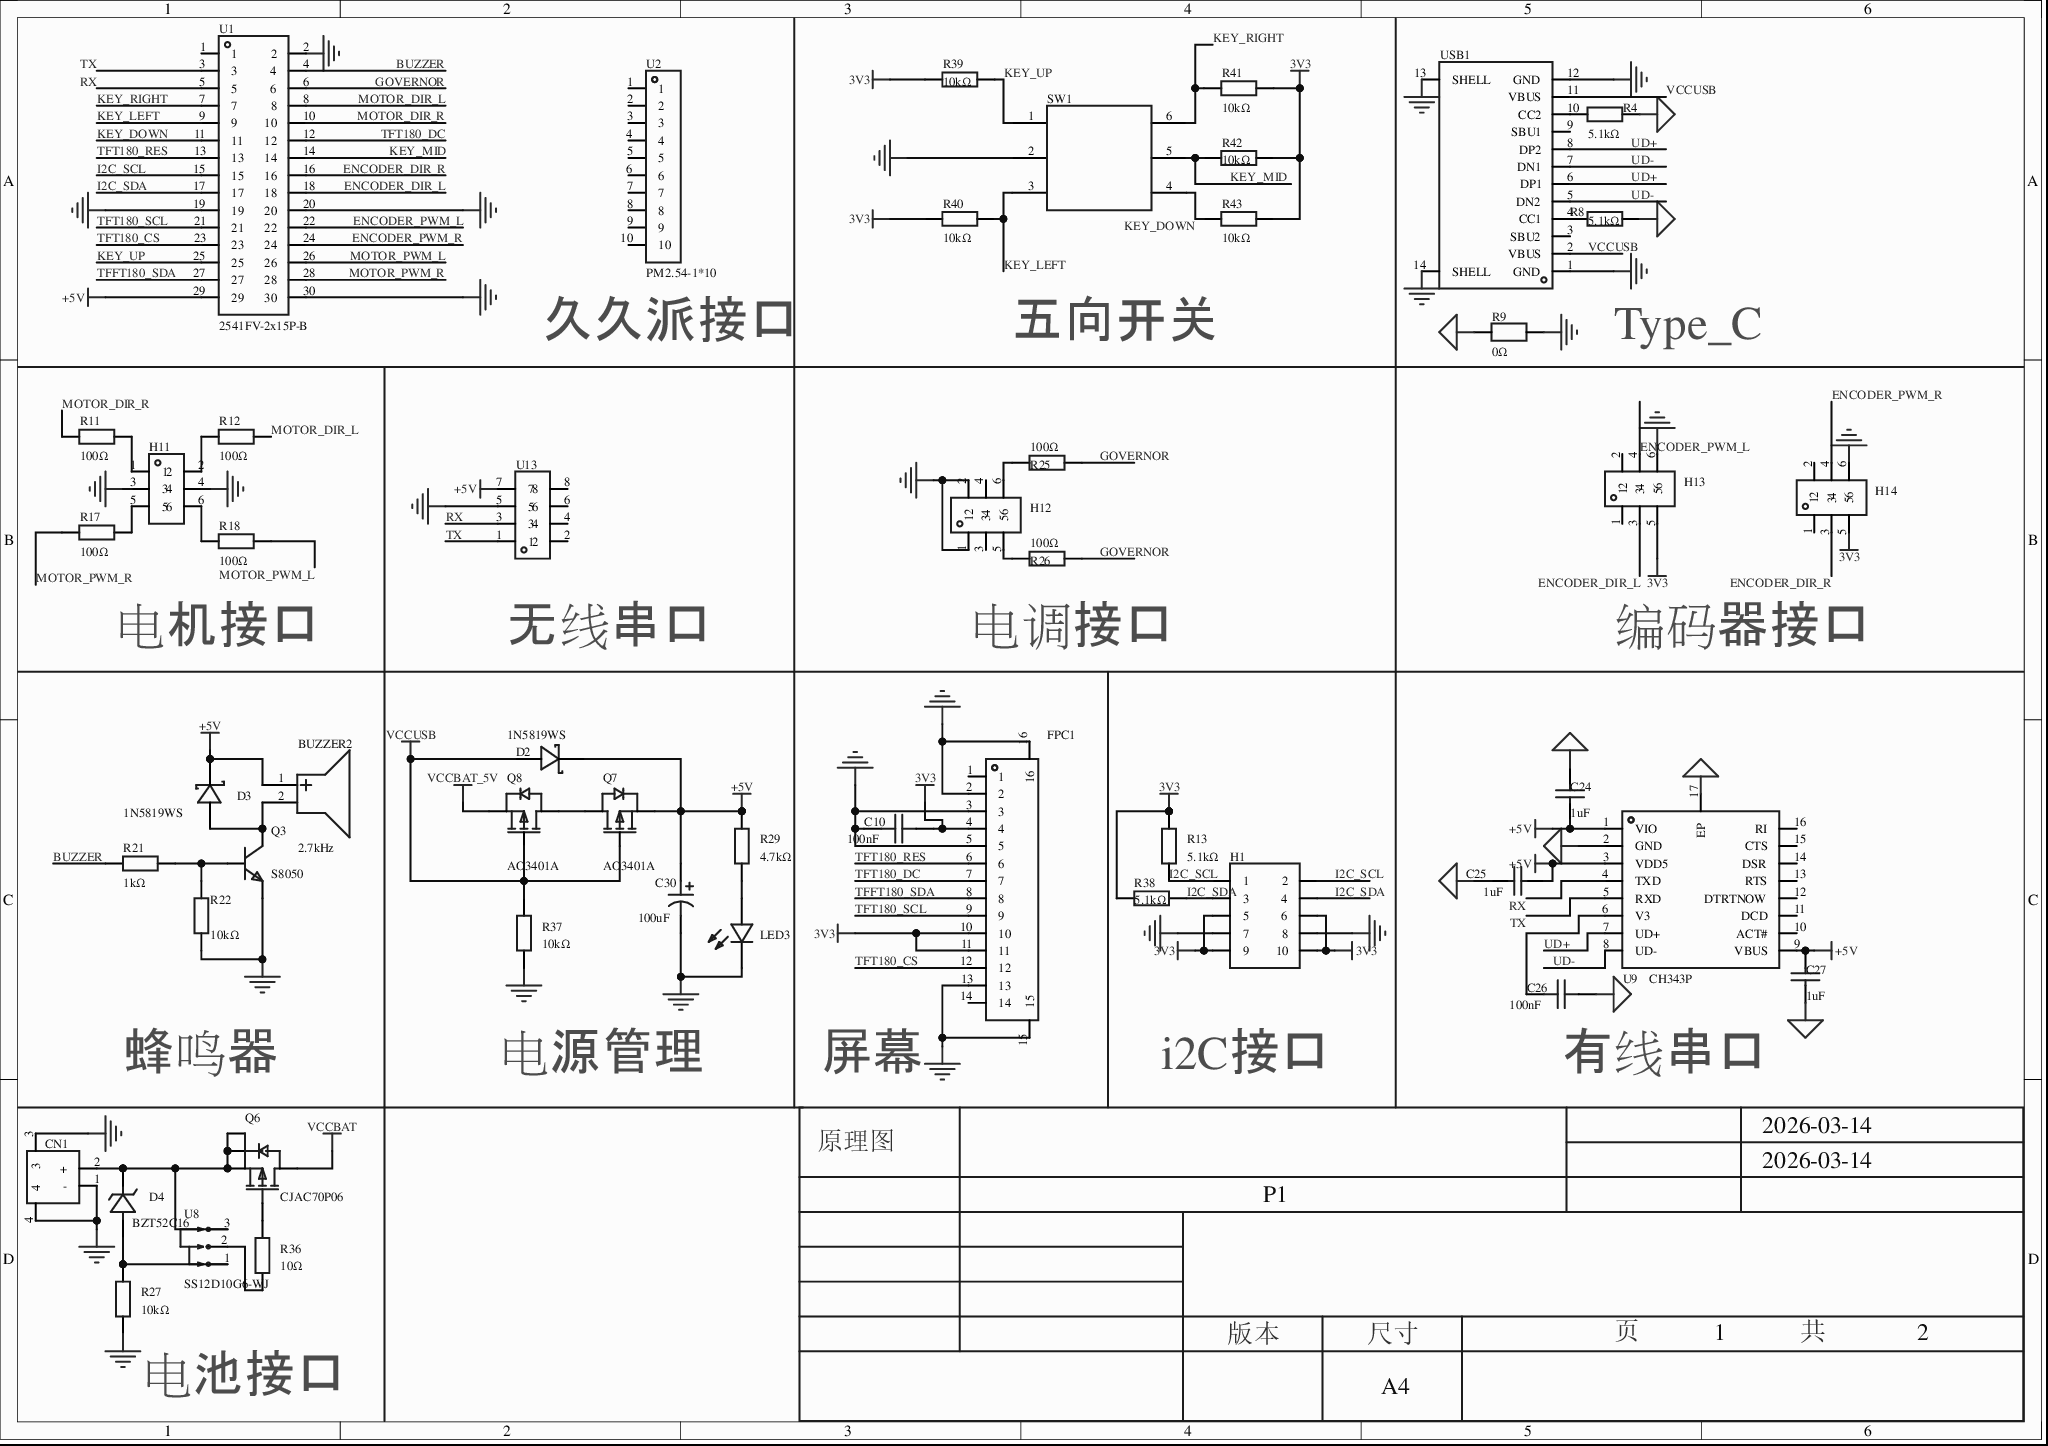
[diagram p0: MISC51977-3.schdoc]
# Altium project MISC51977-2.PrjPcb (part 2 of 2)
## Sheet MISC51977-3.schdoc (continued)
### Library data of the parts (continued)
R36 = 0603WAF100JT5E: 电阻类型:厚膜电阻;阻值:10Ω;精度:±1%;功率:100mW;最大工作电压:75V;温度系数:±400ppm/℃;; Manufacturer: UNI-ROYAL(厚声); AddInBom: yes; ModelId: fc143cca1e79419f9cd78b61e9279f08; ModelTransform: 31.8897,63.7794,0,90,0,0,0,0,0; Tolerance: ±1%; Power(Watts): 100mW; Overload Voltage (Max): 75V; Symbol: 0603WAF100JT5E; Device: 0603WAF100JT5E; LCSC Part Name: 10Ω ±1% 100mW 厚膜电阻; SupplierPart: C22859; ManufacturerPart: 0603WAF100JT5E; Supplier Footprint: 0603; JLCPCB Part Class: 基础库; Datasheet: https://atta.szlcsc.com/upload/public/pdf/source/20200306/C422600_1E6D84923E4A46A82E41ADD87F860B5C.pdf; Supplier: LCSC; ConvertToPcb: yes; FootprintName: R0603; ModelName: R0603; Type: 厚膜电阻; Value: 10Ω; Temperature Coefficient: ±400ppm/℃; Operating Temperature Range: -55℃~+155℃
SW1 = 7*7*5-6P-L WX: 额定电流(DC)：50mA 额定电压(DC)：12V 电路结构：单刀五掷 机械寿命：30000 安装方式：SMD 工作温度：-20℃~+70℃ 开关长度：7.4mm 开关宽度：7.4mm 开关高度：5mm; Manufacturer: SHOU HAN(首韩); AddInBom: yes; ModelId: 64efb118e0fd48f6b5847e0dc15117e6; ModelTransform: 291.338,338.582,0,180,0,0,0,0,-23.622; Symbol: 7*7*5-6P-L WX; Device: 7*7*5-6P-L WX; LCSC Part Name: 7*7*5-6P-L WX; SupplierPart: C2858287; ManufacturerPart: 7*7*5-6P-L WX; Supplier Footprint: SMD-6P,7x7mm; JLCPCB Part Class: 扩展库; Datasheet: https://atta.szlcsc.com/upload/public/pdf/source/20210806/C2858286_484786EF684589807E899A8060F52B6F.pdf; Supplier: LCSC; ConvertToPcb: yes; FootprintName: SW-SMD_8P-L7.0-W7.0-P1.40-LS7.4-TL; ModelName: SW-SMD_8P-L7.0-W7.0-P1.40-LS7.4-TL
U1 = 2541FV-2x15P-B: 插孔结构:2x15P;间距:2.54mm;行距:2.54mm;圆孔/方孔:方孔;安装方式:直插;排数:双排;总孔位数:30P;额定电流:3A;额定电压:-;插孔方向:顶部;塑高:-;触头材质:-;触头镀层:-;工作温度:-40℃~+105℃;; Manufacturer: HanElectricity(瀚源); AddInBom: yes; ModelId: 9476844c889c42239ab5e8be2cdbe540; ModelName: HDR2.54-F-LI-2X15P; ModelTransform: 1499.99708,200,0,0,0,0,0,0,-118.11; Holes Structure: 2x15P; Pitch: 2.54mm; Circular Hole / Square Hole: 方孔; Number of Positions: 30P; Current Rating: 3A; Holes Direction: 顶部; Symbol: 2541FV-2X15P-B; Device: 2541FV-2x15P-B; LCSC Part Name: 2x15P 间距:2.54mm 直插; SupplierPart: C25503127; ManufacturerPart: 2541FV-2x15P-B; Supplier Footprint: 插件,P=2.54mm; JLCPCB Part Class: 扩展库; Datasheet: https://item.szlcsc.com/datasheet/2541FV-2x15P-B/27233670.html; Supplier: LCSC; ConvertToPcb: yes; FootprintName: HDR-TH_30P-P2.54-V-F-R2-C15-S2.54; Row Spacing: 2.54mm; Mounting Type: 直插; Number of Rows: 双排; Voltage Rating (Max): -; Insulation Height: -; Contact Material: -; Contact Plating: -; Operating Temperature: -40℃~+105℃; Supplementary Features: -; PIN Length: -
U2 = PM2.54-1*10: 插孔结构:1x10P;间距:2.54mm;行距:2.54mm;圆孔/方孔:方孔;安装方式:直插;排数:单排;总孔位数:10P;额定电流:2.5A;插孔方向:顶部;塑高:8.5mm;工作温度:-40℃~+105℃;; Manufacturer: ZHOURI(洲日); AddInBom: yes; ModelId: 08a5ee31ec6747838a696d2ac093ffa4; ModelName: HDR-TH_10P-P2.54-F-LI-1X10P; ModelTransform: 1009.87987,100,0,0,0,0,0,0,-125.984; Holes Structure: 1x10P; Pitch: 2.54mm; Circular Hole / Square Hole: 方孔; Number of Positions: 10P; Current Rating: 2.5A; Holes Direction: 顶部; Symbol: PM2.54-1*10; Device: PM2.54-1*10; LCSC Part Name: 间距:2.54mm 1x10P 直插; SupplierPart: C5116489; ManufacturerPart: PM2.54-1*10; Supplier Footprint: 插件,P=2.54mm; JLCPCB Part Class: 扩展库; Datasheet: https://item.szlcsc.com/datasheet/PM2.54-1*10/5692732.html; Supplier: LCSC; ConvertToPcb: yes; FootprintName: HDR-TH_10P-P2.54-V-F; Row Spacing: 2.54mm; Mounting Type: 直插; Number of Rows: 单排; Insulation Height: 8.5mm; Operating Temperature: -40℃~+105℃
U8 = SS12D10G6-WJ: 电路结构:单刀双掷;安装方式:弯插;开关颜色:黑色;额定电流:2A;额定电压:125V;工作寿命:3千次;; Manufacturer: SHOU HAN(首韩); AddInBom: yes; ModelId: a849390df6bd43c0b79d88d5e7a6276e; ModelTransform: 500.3927,685.038,0,0,0,0,0,-317.913,-157.48; Circuit: 单刀双掷; Actuator Style: 矩形柱状; Switch Height: 12.4mm; Actuator Color: 黑色; Current Rating: 2A; Voltage Rating: 125V; Life: 3千次; Symbol: SS12D10G6-WJ; Device: SS12D10G6-WJ; LCSC Part Name: 两档卧式插件 3脚拨动开关弯插 柄长6.0mm; SupplierPart: C7431059; ManufacturerPart: SS12D10G6-WJ; Supplier Footprint: 弯插,12.7x6.7mm; JLCPCB Part Class: 扩展库; Datasheet: https://item.szlcsc.com/datasheet/SS12D10G6-WJ/8431411.html; Supplier: LCSC; ConvertToPcb: yes; FootprintName: SW-TH_3P-P4.80_HX-SS12D10G6-WJ; ModelName: SW-TH_3P-P4.80_HX-SS12D10G6-WJ; Termination Style: PC引脚; Length: 12.7mm; Width: 6.7mm; Mounting Type: 弯插; Operating Temperature: -25℃~+70℃
U9 = CH343P: 应用功能:USB转UART;USB协议版本:USB 2.0;通道数:-;数据速率:6Mbps;; Manufacturer: WCH(南京沁恒); AddInBom: yes; ModelId: bf3177fc8dab4136825cc9ae9b354cf2; ModelTransform: 118.8974,118.8974,0,0,0,0,0,0,0; USB Protocol: USB 2.0; Voltage - Supply: 3.3V；5V; Data Rate: 6Mbps; Symbol: CH343P; Device: CH343P; LCSC Part Name: CH343P; SupplierPart: C2846043; ManufacturerPart: CH343P; Supplier Footprint: TQFN-16-EP(3x3); JLCPCB Part Class: 扩展库; Datasheet: https://item.szlcsc.com/datasheet/CH343P/3039795.html; Supplier: LCSC; ConvertToPcb: yes; FootprintName: TQFN-16_L3.0-W3.0-P0.50-BL-EP1.7; ModelName: TQFN-16_L3.0-W3.0-P0.50-BL-EP1.7; Applications Function: USB转UART; Number of Channels: -; Operating Temperature: -40℃~+85℃
U13 = 5BME8-08872-204-W0: 插孔结构:2x4P;间距:2.54mm;行距:2.54mm;圆孔/方孔:方孔;安装方式:立贴;排数:双排;总孔位数:8P;额定电流:3A;额定电压:-;插孔方向:顶部;塑高:8.5mm;触头材质:黄铜;触头镀层:金;工作温度:-40℃~+105℃;; Manufacturer: SAMZO(三佐); AddInBom: yes; Holes Structure: 2x4P; Pitch: 2.54mm; Circular Hole / Square Hole: 方孔; Number of Positions: 8P; Current Rating: 3A; Holes Direction: 顶部; Symbol: 5BME8-08872-204-W0; Device: 5BME8-08872-204-W0; LCSC Part Name: 2x4P 间距:2.54mm 立贴; SupplierPart: C39832994; ManufacturerPart: 5BME8-08872-204-W0; Supplier Footprint: SMD,P=2.54mm; JLCPCB Part Class: 扩展库; Datasheet: https://item.szlcsc.com/datasheet/5BME8-08872-204-W0/41562139.html; Supplier: LCSC; ConvertToPcb: yes; FootprintName: CONN-SMD_5BME8-08872-204-W0; Row Spacing: 2.54mm; Mounting Type: 立贴; Number of Rows: 双排; Voltage Rating (Max): -; Insulation Height: 8.5mm; Contact Material: 黄铜; Contact Plating: 金; Operating Temperature: -40℃~+105℃
USB1 = TYPE-C 16PIN 2MD(073): 连接器类型:Type-C;标准:USB 3.1;公母:母;安装方式:卧贴;触点数量:16P;端口数量:1;额定电流 - 电源:5A;工作温度范围:-25℃~+85℃;; Manufacturer: SHOU HAN(首韩); AddInBom: yes; ModelId: 3a41b9ec9b654a0fad4d118405ec6290; ModelTransform: 351.9678,298.4246,0,0,0,0,0,-47.244,-35.433; Gender: 母; Number of Contacts: 16P; Number of Ports: 1; Current Rating - Power (Max): 5A; Rated Voltage (Max): 5V; Connect-Disconnect Life: 5千次; Core Colour: 黑色; Symbol: TYPE-C 16PIN 2MD(073); Device: TYPE-C 16PIN 2MD(073); LCSC Part Name: Type-C 母 卧贴; SupplierPart: C2765186; ManufacturerPart: TYPE-C 16PIN 2MD(073); Supplier Footprint: SMD; JLCPCB Part Class: 扩展库; Datasheet: https://atta.szlcsc.com/upload/public/pdf/source/20211123/39B17C16241EAC15C5E277BDA434118E.pdf; Supplier: LCSC; ConvertToPcb: yes; FootprintName: USB-C-SMD_TYPE-C-6PIN-2MD-073; ModelName: USB-C-SMD_TYPE-C-6PIN-2MD-073; Connector Type: Type-C; Standard: USB 3.1; Mounting Style: 卧贴; Operating Temperature Range: -25℃~+85℃

## Sheet MISC51977-4.schdoc
size 297 x 209 mm; Version: V1.0; @Project Name: MISC51977; @Page Count: 2; @Update Date: 2026-03-14; @Create Date: 2026-03-14; @Schematic Name: MISC51977; @Page No: 2; @Board Name: MISC51977; @Create Time: 16:06:18; @Update Time: 17:32:11
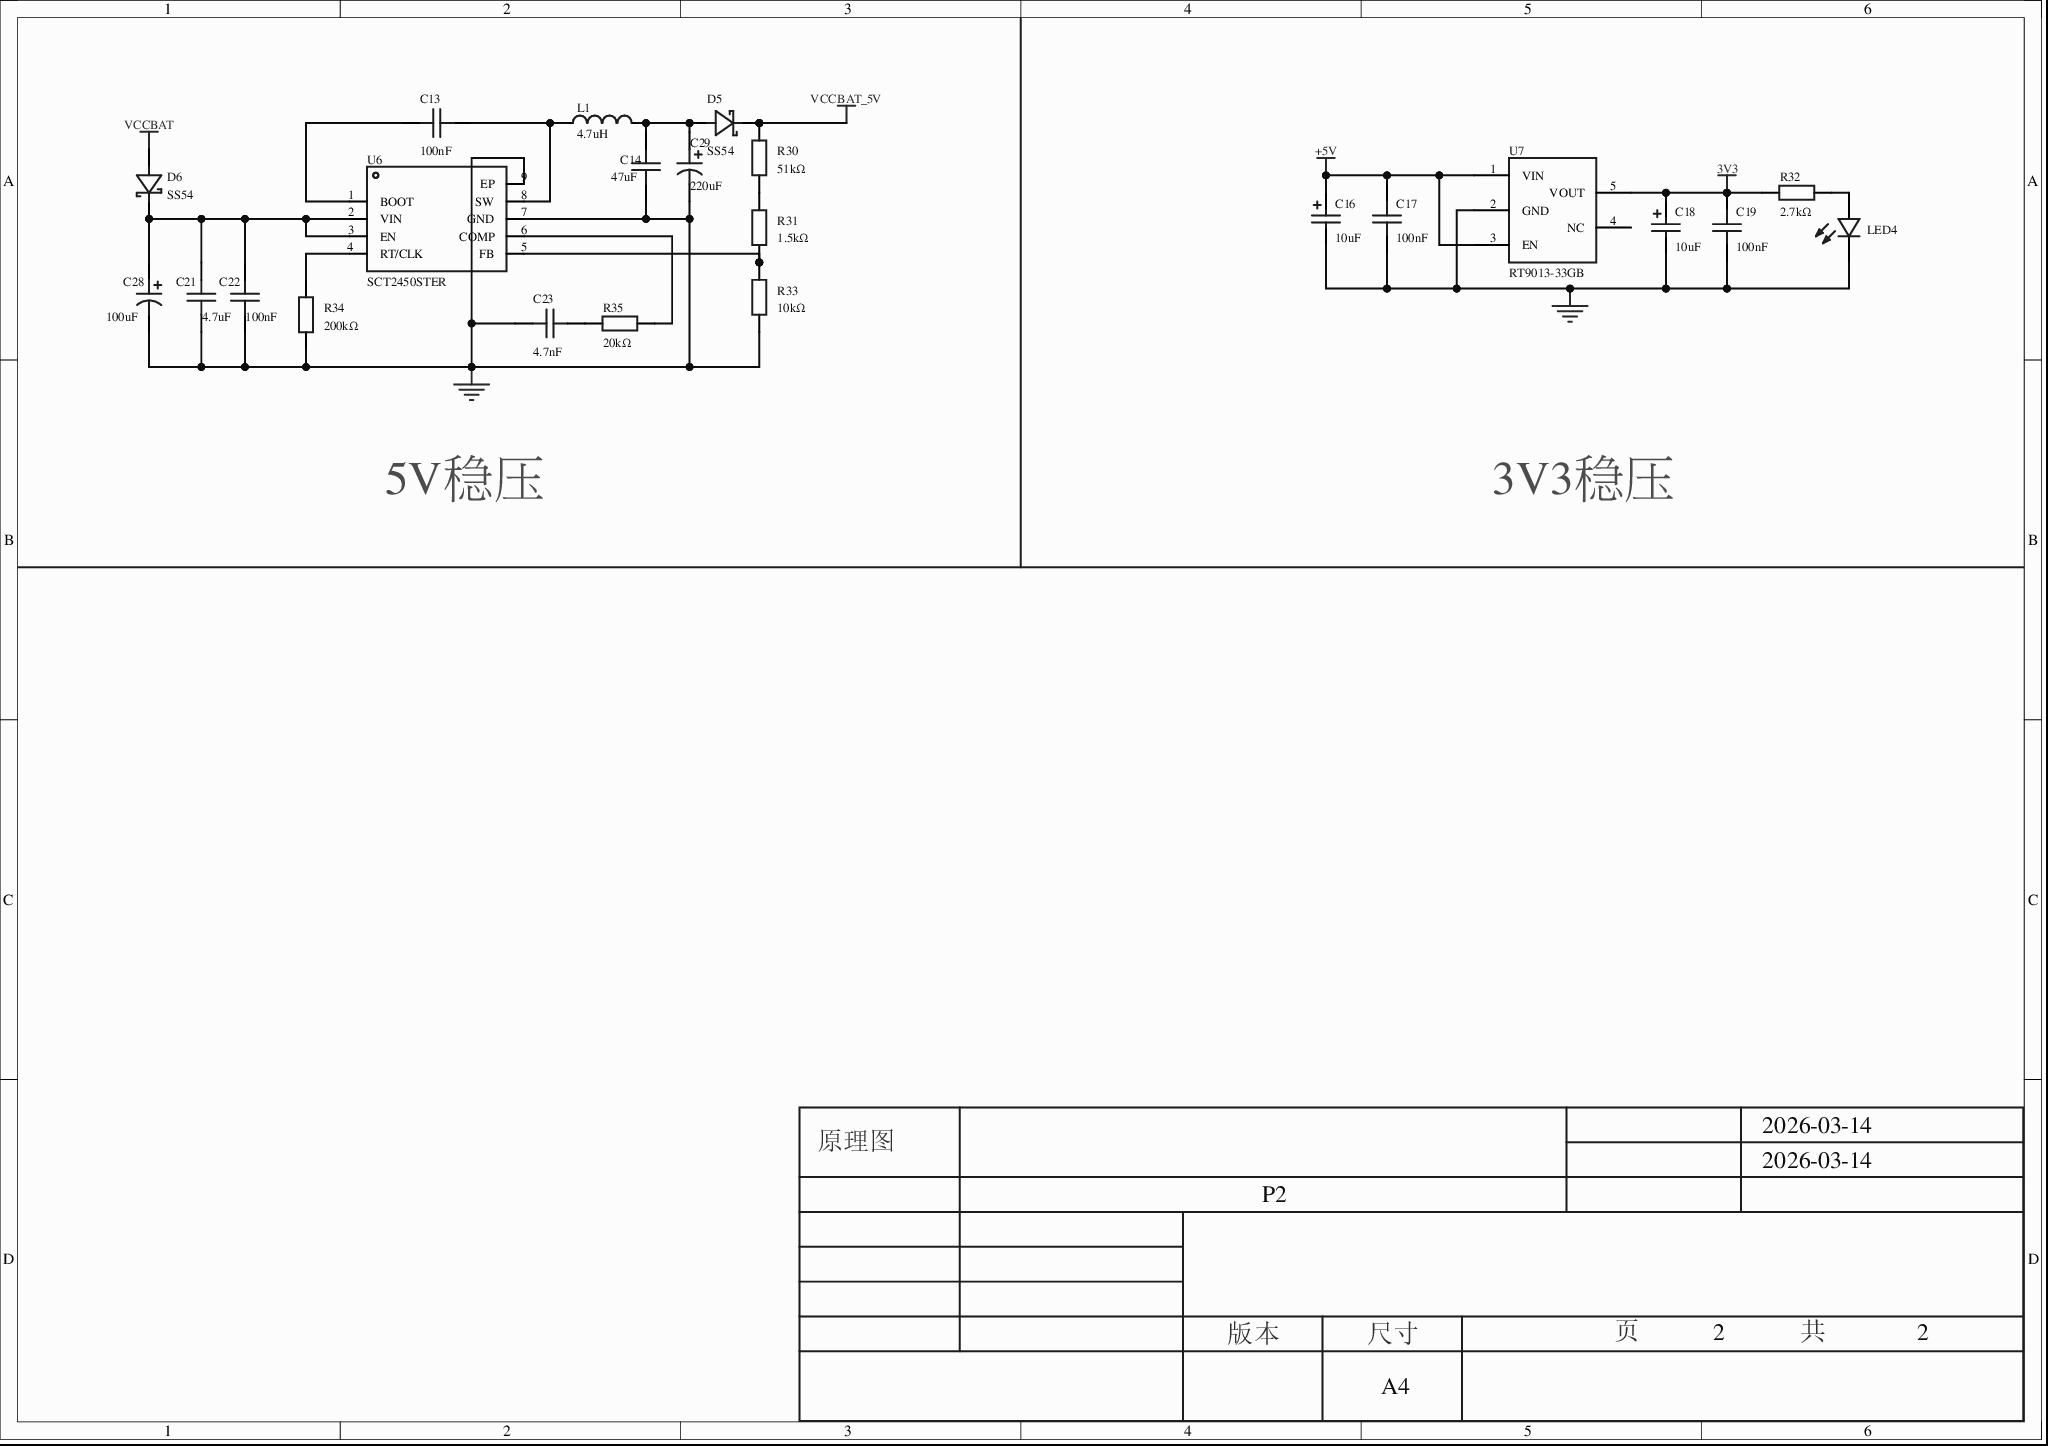
[diagram p1: MISC51977-4.schdoc]

### Parts
C13  100nF  [C0603]
C14  47uF  [C1206]
C16  10uF  [CAP-SMD_L3.2-W1.6-RD-C7171]
C17  100nF  [C0603]
C18  10uF  [CAP-SMD_L3.2-W1.6-RD-C7171]
C19  100nF  [C0603]
C21  4.7uF  [C1206]
C22  100nF  [C0603]
C23  4.7nF  [C0603]
C28  100uF  [CAP-SMD_BD6.3-L6.6-W6.6-FD-1]
C29  220uF  [CAP-SMD_BD6.3-L6.6-W6.6-LS7.3-FD-H7.7]
D5  SS54  [SMA_L4.3-W2.6-LS5.0-FD]
D6  SS54  [SMA_L4.3-W2.6-LS5.0-FD]
L1  4.7uH  [IND-SMD_L5.4-W5.2_FXL0530]
LED4  NCD0603R1  [LED0603-RD_RED]  (value not drawn)
R30  51kΩ  [R0603]
R31  1.5kΩ  [R0603]
R32  2.7kΩ  [R0603]
R33  10kΩ  [R0603]
R34  200kΩ  [R0603]
R35  20kΩ  [R0603]
U6  SCT2450STER  [ESOP-8_L4.9-W3.9-P1.27-LS6.0-BL-EP]
U7  RT9013-33GB  [SOT-23-5_L3.0-W1.7-P0.95-LS2.8-BL]

### Nets
3V3: C18.1 C19.1 R32.1 U7.5(VOUT)
+5V: C16.1 C17.1 U7.1(VIN) U7.3(EN)
GND: C14.1 C16.2 C17.2 C18.2 C19.2 C21.1 C22.1 C23.1 C28.2 C29.2 LED4.1(K) R33.1 R34.1 U6.7(GND) U6.9(EP) U7.2(GND)
VCCBAT: D6.1(A)
VCCBAT_5V: D5.2(K) R30.2
NetC13_1: C13.1 L1.1 U6.8(SW)
NetC13_2: C13.2 U6.1(BOOT)
NetC14_2: C14.2 C29.1 D5.1(A) L1.2
NetC21_2: C21.2 C22.2 C28.1 D6.2(K) U6.2(VIN) U6.3(EN)
NetC23_2: C23.2 R35.1
NetLED4_2: LED4.2(A) R32.2
NetR30_1: R30.1 R31.2
NetR31_1: R31.1 R33.2 U6.5(FB)
NetR34_2: R34.2 U6.4(RT/CLK)
NetR35_2: R35.2 U6.6(COMP)

Not connected (* = marked no-connect by the designer): U7 4(NC)*

### Notes on the sheet
- 5V稳压
- 3V3稳压
- 2026-03-14
- 原理图
- P2
- 版本
- 尺寸
- A4
- 页
- 2
- 共

### Library data of the parts
C13 C17 C19 C22 = CGA0603X7R104K500JT: as C10 on sheet MISC51977-3; Symbol: CGA0603X7R104K500JT; Device: CGA0603X7R104K500JT; LCSC Part Name: 100nF ±10% 50V; SupplierPart: C6119867; ManufacturerPart: CGA0603X7R104K500JT; Supplier Footprint: 0603; JLCPCB Part Class: 扩展库; Supplier: LCSC; ConvertToPcb: yes; FootprintName: C0603; Value: 100nF
C14 = CGA1206X5R476M250NT: 容值:47uF;精度:±20%;额定电压:25V;材质(温度系数):X5R;; Manufacturer: HRE(芯声); AddInBom: yes; ModelId: e4be705b945545a48e666415e3682bd8; ModelName: C1206_L3.2-W1.6-H1.3; ModelTransform: 125.984,62.992,0,0,0,0,0,0,0; Tolerance: ±20%; Voltage Rated: 25V; Temperature Coefficient: X5R; Symbol: CGA1206X5R476M250NT; Device: CGA1206X5R476M250NT; LCSC Part Name: 47uF ±20% 25V; SupplierPart: C6119973; ManufacturerPart: CGA1206X5R476M250NT; Supplier Footprint: 1206; JLCPCB Part Class: 扩展库; Datasheet: https://atta.szlcsc.com/upload/public/pdf/source/20240229/85D0248657B5565B358B20AFC8F32D04.pdf; Supplier: LCSC; ConvertToPcb: yes; FootprintName: C1206; Value: 47uF
C16 C18 = TAJA106K016RNJ: 容值:10uF;精度:±10%;额定电压:16V;等效串联电阻:3Ω@100kHz;; Manufacturer: Kyocera AVX; AddInBom: yes; ModelId: d42b6f9952ad429a883ac5dd55ff7452; ModelName: CASE-A_L3.2-W1.6-H1.6; ModelTransform: 125.984,62.992,0,0,0,0,0,0,0; Tolerance: ±10%; Rated Voltage: 16V; Symbol: TAJA106K016RNJ; Device: TAJA106K016RNJ; LCSC Part Name: 10uF ±10% 16V; SupplierPart: C7171; ManufacturerPart: TAJA106K016RNJ; Supplier Footprint: CASE-A-3216; JLCPCB Part Class: 基础库; Datasheet: https://atta.szlcsc.com/upload/public/pdf/source/20160107/1457707750344.pdf; Supplier: LCSC; ConvertToPcb: yes; FootprintName: CAP-SMD_L3.2-W1.6-RD-C7171; Value: 10uF; Equivalent Series Resistance(ESR): 3Ω@100kHz; Operating Temperature: -55℃~+125℃
C21 = CGA1206X5R475K350NT: 容值:4.7uF;精度:±10%;额定电压:35V;材质(温度系数):X5R;; Manufacturer: HRE(芯声); AddInBom: yes; ModelId: e4be705b945545a48e666415e3682bd8; ModelName: C1206_L3.2-W1.6-H1.3; ModelTransform: 125.984,62.992,0,0,0,0,0,0,0; Tolerance: ±10%; Voltage Rating: 35V; Temperature Coefficient: X5R; Symbol: CGA1206X5R475K350NT; Device: CGA1206X5R475K350NT; LCSC Part Name: 4.7uF ±10% 35V; SupplierPart: C22399656; ManufacturerPart: CGA1206X5R475K350NT; Supplier Footprint: 1206; JLCPCB Part Class: 扩展库; Datasheet: https://atta.szlcsc.com/upload/public/pdf/source/20240523/B8FD0004515F911A9E977ED73F0FE1A1.pdf; Supplier: LCSC; ConvertToPcb: yes; FootprintName: C1206; Value: 4.7uF
C23 = CGA0603X7R472K500JT: 容值:4.7nF;精度:±10%;额定电压:50V;材质(温度系数):X7R;; Manufacturer: HRE(芯声); AddInBom: yes; ModelId: ac125912035d415993ca9572d50418b1; ModelName: C0603_L1.6-W0.8-H0.8; ModelTransform: 62.992,31.496,0,0,0,0,0,0,0; Tolerance: ±10%; Voltage Rated: 50V; Temperature Coefficient: X7R; Symbol: CGA0603X7R472K500JT; Device: CGA0603X7R472K500JT; LCSC Part Name: 4.7nF ±10% 50V; SupplierPart: C7503499; ManufacturerPart: CGA0603X7R472K500JT; Supplier Footprint: 0603; JLCPCB Part Class: 扩展库; Supplier: LCSC; ConvertToPcb: yes; FootprintName: C0603; Value: 4.7nF
C28 = JVJ25V100M6x5: as C30 on sheet MISC51977-3; Symbol: JVJ25V100M6X5; Device: JVJ25V100M6x5; LCSC Part Name: 100uF ±20% 25V; SupplierPart: C46550402; ManufacturerPart: JVJ25V100M6x5; Supplier Footprint: SMD,D6.3xL5.4mm; JLCPCB Part Class: 扩展库; Datasheet: https://item.szlcsc.com/datasheet/JVJ25V100M6x5/48680096.html; Supplier: LCSC; ConvertToPcb: yes; FootprintName: CAP-SMD_BD6.3-L6.6-W6.6-FD-1; ModelName: CAP-SMD_BD6.3-L6.6-W6.6-FD-1; Value: 100uF; Ripple Current: 72mA@120Hz; Diameter: 6.3mm; Height - Seated (Max): 5.4mm; Operating Temperature: -55℃~+105℃
C29 = JVJ25V220M6x8: 容值:220uF;精度:±20%;额定电压:25V;纹波电流:120mA@120Hz;; Manufacturer: JIERR(捷而瑞); AddInBom: yes; ModelId: ccbda52dceed4b139172c40f75c9da3f; ModelTransform: 287.401,259.842,0,0,0,0,0,0,0; Tolerance: ±20%; Voltage Rating: 25V; Lifetime: 2000hrs@105℃; Symbol: JVJ25V220M6X8; Device: JVJ25V220M6x8; LCSC Part Name: 220uF ±20% 25V; SupplierPart: C46550404; ManufacturerPart: JVJ25V220M6x8; Supplier Footprint: SMD,D6.3xL7.7mm; JLCPCB Part Class: 扩展库; Datasheet: https://item.szlcsc.com/datasheet/JVJ25V220M6x8/48680098.html; Supplier: LCSC; ConvertToPcb: yes; FootprintName: CAP-SMD_BD6.3-L6.6-W6.6-LS7.3-FD-H7.7; ModelName: CAP-SMD_BD6.3-L6.6-W6.6-LS7.3-FD-H7.7; Value: 220uF; Ripple Current: 120mA@120Hz; Diameter: 6.3mm; Height - Seated (Max): 7.7mm; Operating Temperature: -55℃~+105℃
D5 D6 = SS54_C7420369: 二极管配置:独立式;正向压降(Vf):550mV@5.0A;直流反向耐压(Vr):40V;整流电流:5A;; Manufacturer: 宏迦橙; AddInBom: yes; ModelId: 7e24bebe6cd74171ae8c9de6fc5b78aa; ModelTransform: 198.4248,103.5431,0,180,0,0,0,0,0; Diode Configuration: 独立式; Reverse Voltage (Vr): 40V; Rectified Current: 5A; Reverse Leakage Current (Ir): 50uA@40V; Symbol: SS54_C7420369; Device: SS54_C7420369; LCSC Part Name: 电压:40V 电流:5A; SupplierPart: C7420369; ManufacturerPart: SS54; Supplier Footprint: SMA(DO-214AC); JLCPCB Part Class: 扩展库; Datasheet: https://atta.szlcsc.com/upload/public/pdf/source/20230828/254C3882F8647358AD9F60DD73611B5E.pdf; Supplier: LCSC; ConvertToPcb: yes; FootprintName: SMA_L4.3-W2.6-LS5.0-FD; ModelName: SMA_L4.3-W2.6-LS5.0-FD; Forward Voltage (Vf@If): 550mV@5.0A
L1 = FXL0530-4R7-M: 电感值:4.7uH;精度:±20%;额定电流:4.5A;饱和电流(Isat):5A;类型:一体成型电感;; Manufacturer: cjiang(长江微电); AddInBom: yes; ModelId: e41ad6dce8434108a9c5d36a52ebad3b; ModelName: IND-SMD_L5.4-W5.2-H2.8_FXL0530; ModelTransform: 212.598,204.724,0,0,0,0,0,0,0; Tolerance: ±20%; Rated Current: 4.5A; Saturation Current (Isat): 5A; DC Resistance (DCR): 60mΩ; Type: 一体成型电感; Symbol: FXL0530-4R7-M; Device: FXL0530-4R7-M; LCSC Part Name: 4.7uH ±20% 5A; SupplierPart: C177246; ManufacturerPart: FXL0530-4R7-M; Supplier Footprint: SMD,5.2x5.4mm; JLCPCB Part Class: 扩展库; Datasheet: https://atta.szlcsc.com/upload/public/pdf/source/20240426/3189EA8206330E2108542F9E34E540E7.pdf; Supplier: LCSC; ConvertToPcb: yes; FootprintName: IND-SMD_L5.4-W5.2_FXL0530; Value: 4.7uH
LED4 = NCD0603R1_C84263: as LED3 on sheet MISC51977-3; Device: NCD0603R1_C84263; LCSC Part Name: NCD0603R1; SupplierPart: C84263; ManufacturerPart: NCD0603R1; Supplier Footprint: 0603; JLCPCB Part Class: 扩展库; Datasheet: https://atta.szlcsc.com/upload/public/pdf/source/20200820/C84263_DABC6A75E58F576973B407FDBA283D60.pdf; Supplier: LCSC; ConvertToPcb: yes; FootprintName: LED0603-RD_RED; ModelName: LED0603-RD_RED; Lamp Holder Type: -; Forward Voltage (VF): 1.6V~2.6V; Dominant Wavelength: 615nm~630nm; Peak Wavelength: -; Color Temperature: -; Luminous Intensity: 80mcd~220mcd; Mounting Sytle: -; Operating Temperature: -30℃~+85℃
R30 = 0603WAF5102T5E: 电阻类型:厚膜电阻;阻值:51kΩ;精度:±1%;功率:100mW;最大工作电压:75V;温度系数:±100ppm/℃;; Manufacturer: UNI-ROYAL(厚声); AddInBom: yes; ModelId: fc143cca1e79419f9cd78b61e9279f08; ModelTransform: 31.8897,63.7794,0,90,0,0,0,0,0; Tolerance: ±1%; Power(Watts): 100mW; Overload Voltage (Max): 75V; Symbol: 0603WAF5102T5E; Device: 0603WAF5102T5E; LCSC Part Name: 51kΩ ±1% 100mW 厚膜电阻; SupplierPart: C23196; ManufacturerPart: 0603WAF5102T5E; Supplier Footprint: 0603; JLCPCB Part Class: 基础库; Datasheet: https://atta.szlcsc.com/upload/public/pdf/source/20200306/C422600_1E6D84923E4A46A82E41ADD87F860B5C.pdf; Supplier: LCSC; ConvertToPcb: yes; FootprintName: R0603; ModelName: R0603; Type: 厚膜电阻; Value: 51kΩ; Temperature Coefficient: ±100ppm/℃; Operating Temperature Range: -55℃~+155℃
R31 = 0603WAF1501T5E: 电阻类型:厚膜电阻;阻值:1.5kΩ;精度:±1%;功率:100mW;最大工作电压:75V;温度系数:±100ppm/℃;; Manufacturer: UNI-ROYAL(厚声); AddInBom: yes; ModelId: fc143cca1e79419f9cd78b61e9279f08; ModelTransform: 31.8897,63.7794,0,90,0,0,0,0,0; Tolerance: ±1%; Power(Watts): 100mW; Overload Voltage (Max): 75V; Symbol: 0603WAF1501T5E; Device: 0603WAF1501T5E; LCSC Part Name: 1.5kΩ ±1% 100mW 厚膜电阻; SupplierPart: C22843; ManufacturerPart: 0603WAF1501T5E; Supplier Footprint: 0603; JLCPCB Part Class: 基础库; Datasheet: https://atta.szlcsc.com/upload/public/pdf/source/20200306/C422600_1E6D84923E4A46A82E41ADD87F860B5C.pdf; Supplier: LCSC; ConvertToPcb: yes; FootprintName: R0603; ModelName: R0603; Type: 厚膜电阻; Value: 1.5kΩ; Temperature Coefficient: ±100ppm/℃; Operating Temperature Range: -55℃~+155℃
R32 = 0603WAF2701T5E: 电阻类型:厚膜电阻;阻值:2.7kΩ;精度:±1%;功率:100mW;最大工作电压:75V;温度系数:±100ppm/℃;; Manufacturer: UNI-ROYAL(厚声); AddInBom: yes; ModelId: fc143cca1e79419f9cd78b61e9279f08; ModelTransform: 31.8897,63.7794,0,90,0,0,0,0,0; Tolerance: ±1%; Power(Watts): 100mW; Overload Voltage (Max): 75V; Symbol: 0603WAF2701T5E; Device: 0603WAF2701T5E; LCSC Part Name: 2.7kΩ ±1% 100mW 厚膜电阻; SupplierPart: C13167; ManufacturerPart: 0603WAF2701T5E; Supplier Footprint: 0603; JLCPCB Part Class: 基础库; Datasheet: https://atta.szlcsc.com/upload/public/pdf/source/20200306/C422600_1E6D84923E4A46A82E41ADD87F860B5C.pdf; Supplier: LCSC; ConvertToPcb: yes; FootprintName: R0603; ModelName: R0603; Type: 厚膜电阻; Value: 2.7kΩ; Temperature Coefficient: ±100ppm/℃; Operating Temperature Range: -55℃~+155℃
R33 = 0603WAF1002T5E: as R22 on sheet MISC51977-3; Symbol: 0603WAF1002T5E; Device: 0603WAF1002T5E; LCSC Part Name: 厚膜电阻 10kΩ ±1% 100mW; SupplierPart: C25804; ManufacturerPart: 0603WAF1002T5E; Supplier Footprint: 0603; JLCPCB Part Class: 基础库; Datasheet: https://atta.szlcsc.com/upload/public/pdf/source/20200306/C422600_1E6D84923E4A46A82E41ADD87F860B5C.pdf; Supplier: LCSC; ConvertToPcb: yes; FootprintName: R0603; ModelName: R0603; Type: 厚膜电阻; Value: 10kΩ; Temperature Coefficient: ±100ppm/℃; Operating Temperature Range: -55℃~+155℃
R34 = 0603WAF2003T5E: 电阻类型:厚膜电阻;阻值:200kΩ;精度:±1%;功率:100mW;最大工作电压:75V;温度系数:±100ppm/℃;; Manufacturer: UNI-ROYAL(厚声); AddInBom: yes; ModelId: fc143cca1e79419f9cd78b61e9279f08; ModelTransform: 31.8897,63.7794,0,90,0,0,0,0,0; Tolerance: ±1%; Power(Watts): 100mW; Overload Voltage (Max): 75V; Symbol: 0603WAF2003T5E; Device: 0603WAF2003T5E; LCSC Part Name: 200kΩ ±1% 100mW 厚膜电阻; SupplierPart: C25811; ManufacturerPart: 0603WAF2003T5E; Supplier Footprint: 0603; JLCPCB Part Class: 基础库; Datasheet: https://atta.szlcsc.com/upload/public/pdf/source/20200306/C422600_1E6D84923E4A46A82E41ADD87F860B5C.pdf; Supplier: LCSC; ConvertToPcb: yes; FootprintName: R0603; ModelName: R0603; Type: 厚膜电阻; Value: 200kΩ; Temperature Coefficient: ±100ppm/℃; Operating Temperature Range: -55℃~+155℃
R35 = 0603WAF2002T5E: 电阻类型:厚膜电阻;阻值:20kΩ;精度:±1%;功率:100mW;最大工作电压:75V;温度系数:±100ppm/℃;; Manufacturer: UNI-ROYAL(厚声); AddInBom: yes; ModelId: fc143cca1e79419f9cd78b61e9279f08; ModelTransform: 31.8897,63.7794,0,90,0,0,0,0,0; Tolerance: ±1%; Power(Watts): 100mW; Overload Voltage (Max): 75V; Symbol: 0603WAF2002T5E; Device: 0603WAF2002T5E; LCSC Part Name: 20kΩ ±1% 100mW 厚膜电阻; SupplierPart: C4184; ManufacturerPart: 0603WAF2002T5E; Supplier Footprint: 0603; JLCPCB Part Class: 基础库; Datasheet: https://atta.szlcsc.com/upload/public/pdf/source/20200306/C422600_1E6D84923E4A46A82E41ADD87F860B5C.pdf; Supplier: LCSC; ConvertToPcb: yes; FootprintName: R0603; ModelName: R0603; Type: 厚膜电阻; Value: 20kΩ; Temperature Coefficient: ±100ppm/℃; Operating Temperature Range: -55℃~+155℃
U6 = SCT2450STER: 功能类型:降压型;工作电压:3.8V~36V;输出电流:5A;; Manufacturer: SCT(芯洲科技); AddInBom: yes; ModelId: d3e00daa36c445139c055a3b9efb85d2; ModelName: ESOP-8_L4.9-W3.9-H1.6-LS6.0-P1.27; ModelTransform: 240.157,192.913,0,90,0,0,0,0,0; Function: 降压型; Output Current: 5A; Switching Frequency: 100kHz~1.1MHz; Synchronous Rectification: 是; Number of Outputs: 1; Switch tube (built-in/external): 内置; Symbol: SCT2450STER; Device: SCT2450STER; LCSC Part Name: 3.8V-36V输入，5A输出，高效率同步降压DC-DC转换器; SupplierPart: C509400; ManufacturerPart: SCT2450STER; Supplier Footprint: ESOP-8; JLCPCB Part Class: 扩展库; Datasheet: https://atta.szlcsc.com/upload/public/pdf/source/20200407/C509400_EDF779A672A59398CFBA9E95FA584FEC.pdf; Supplier: LCSC; ConvertToPcb: yes; FootprintName: ESOP-8_L4.9-W3.9-P1.27-LS6.0-BL-EP; Input Voltage: 3.8V~36V; Operating Temperature: -40℃~+125℃@(TJ)
U7 = RT9013-33GB: 输出类型:固定;最大输入电压:5.5V;输出电压:3.3V;输出电流:500mA;电源纹波抑制比(PSRR):50dB@(10kHz);输出极性:正极;; Manufacturer: RICHTEK(立锜); AddInBom: yes; ModelId: 0a2a1b8f50944f73965918ad6e5fe167; ModelName: SOT-23-5_L2.9-W1.6-H1.1-LS2.8-P0.95; ModelTransform: 118.60433,114.173,0,90,0,0,0.0005,0.0005,0; Output Type: 固定; Maximum Input Voltage: 5.5V; Output Voltage: 3.3V; Output Current: 500mA; Dropout Voltage: 400mV@(500mA); standby current: 50uA; Output Polarity: 正极; Number of Outputs: 1; Symbol: RT9013-33GB; Device: RT9013-33GB; LCSC Part Name: 输入5.5V 输出3.3V 500mA; SupplierPart: C47773; ManufacturerPart: RT9013-33GB; Supplier Footprint: SOT-23-5; JLCPCB Part Class: 扩展库; Datasheet: https://atta.szlcsc.com/upload/public/pdf/source/20150504/1457707282459.pdf; Supplier: LCSC; ConvertToPcb: yes; FootprintName: SOT-23-5_L3.0-W1.7-P0.95-LS2.8-BL; Power Supply Rejection Ratio (PSRR): 50dB@(10kHz); Noise: -; Feature: 低ESR；防静电保护；热保护(TSD)；过流保护(OCP)；带使能; Operating Temperature: -40℃~+85℃

## Nets that join several sheets
3V3: MISC51977-3 (17 pins), MISC51977-4 (C18.1 C19.1 R32.1 U7.5)
+5V: MISC51977-3 (14 pins), MISC51977-4 (C16.1 C17.1 U7.1 U7.3)
GND: MISC51977-3 (35 pins), MISC51977-4 (16 pins)
VCCBAT: MISC51977-3 (Q6.5), MISC51977-4 (D6.1)
VCCBAT_5V: MISC51977-3 (Q8.2), MISC51977-4 (D5.2 R30.2)